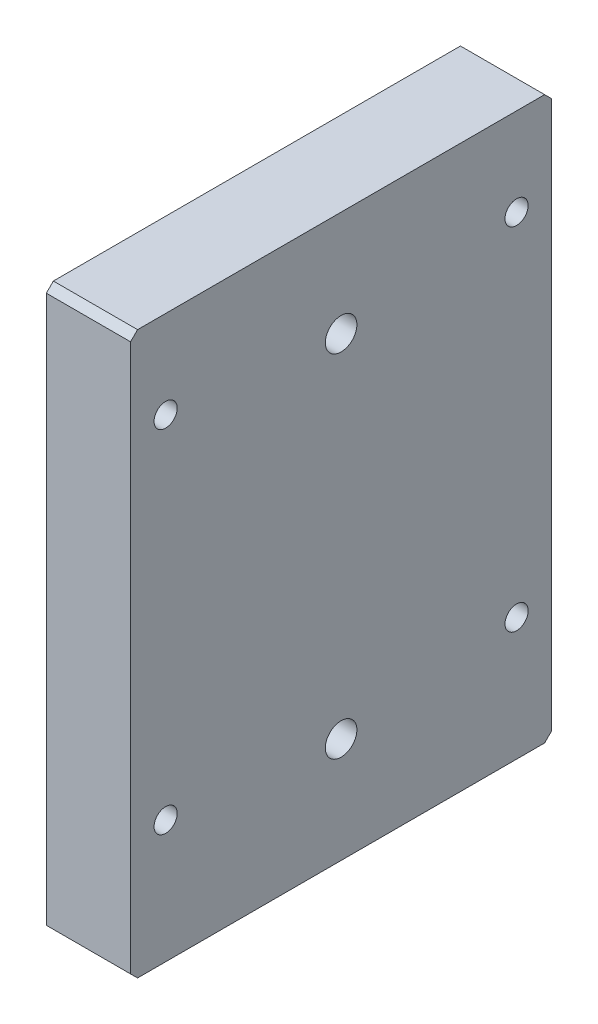
SolidWorks part; units mm, degrees
material "AL6061"
ref_plane "Front Plane" through (0, 0, 0) normal (0, 0, 1) x (1, 0, 0)
ref_plane "Top Plane" through (0, 0, 0) normal (0, 1, 0) x (1, 0, 0)
ref_plane "Right Plane" through (0, 0, 0) normal (1, 0, 0) x (0, 0, -1)
sketch "Sketch1" plane through (0, 0, 0) normal (1, 0, 0) x (0, 0, -1)
  line L1 (-30, -40) -> (30, -40)
  line L2 (-30, -40) -> (-30, 40)
  line L3 (-30, 40) -> (30, 40)
  line L4 (30, -40) -> (30, 40)
  line L5 (-30, -40) -> (30, 40) construction
  line L6 (-30, 40) -> (30, -40) construction
  point P0 (0, 0)
  dimension "D1" = 60
  dimension "D2" = 80
extrude "Boss-Extrude1" add sketch "Sketch1" along normal blind 12
hole_wizard "M4 Tapped Hole1" positions "Sketch2" profile "Sketch3" tap size "M4" standard "GB" end condition through all
sketch "Sketch2" plane through (0, 0, 0) normal (-1, 0, 0) x (0, 0, 1)
  point P0 (-25, 27.5)
  point P3 (-25, -22.5)
  point P6 (25, -22.5)
  point P9 (25, 27.5)
cosmetic thread "Cosmetic thread1" parameters "D2"=4
cosmetic thread "Cosmetic thread2" parameters "D2"=4
cosmetic thread "Cosmetic thread3" parameters "D2"=4
cosmetic thread "Cosmetic thread4" parameters "D2"=4
sketch "Sketch3" plane through (0, 27.5, -25) normal (0, 1, 0) x (0, 0, 1)
  line L0 (0, 0) -> (0, 12)
  line L1 (0, 12) -> (1.65, 12)
  line L2 (1.65, 12) -> (1.65, 0)
  line L5 (1.65, 0) -> (0, 0)
  line L11 (0, -6.35) -> (0, 107.95) construction
  dimension "通孔螺纹孔钻头直径" = 3.3
  dimension "通孔螺纹孔钻头深度" = 12
hole_wizard "CBORE for M4 Hexagon socket head cap screws1" positions "Sketch4" profile "Sketch5" counterbore size "M4" standard "GB" end condition through all
sketch "Sketch4" plane through (0, 0, 0) normal (-1, 0, 0) x (0, 0, 1)
  line L0 (0, 0) -> (30, 0) construction
  line L1 (30, 40) -> (30, -40) construction
  point P0 (0, -25)
  point P2 (0, 25)
  dimension "D1" = 50
sketch "Sketch5" plane through (0, -25, 0) normal (0, 1, 0) x (0, 0, 1)
  line L0 (0, 0) -> (0, 12)
  line L1 (0, 12) -> (2.25, 12)
  line L3 (2.25, 12) -> (2.25, 4.6)
  line L4 (2.25, 4.6) -> (4, 4.6)
  line L5 (4, 4.6) -> (4, 0)
  line L7 (4, 0) -> (0, 0)
  line L11 (0, -6.35) -> (0, 107.95) construction
  dimension "通孔孔直径" = 4.5
  dimension "通孔孔深度" = 12
  dimension "柱形沉头孔直径" = 8
  dimension "柱形沉头孔深度" = 4.6
chamfer "Chamfer1" distance 1 angle 45 4 edges at (6, -40, -30) (6, 40, -30) (6, -40, 30) (6, 40, 30)
